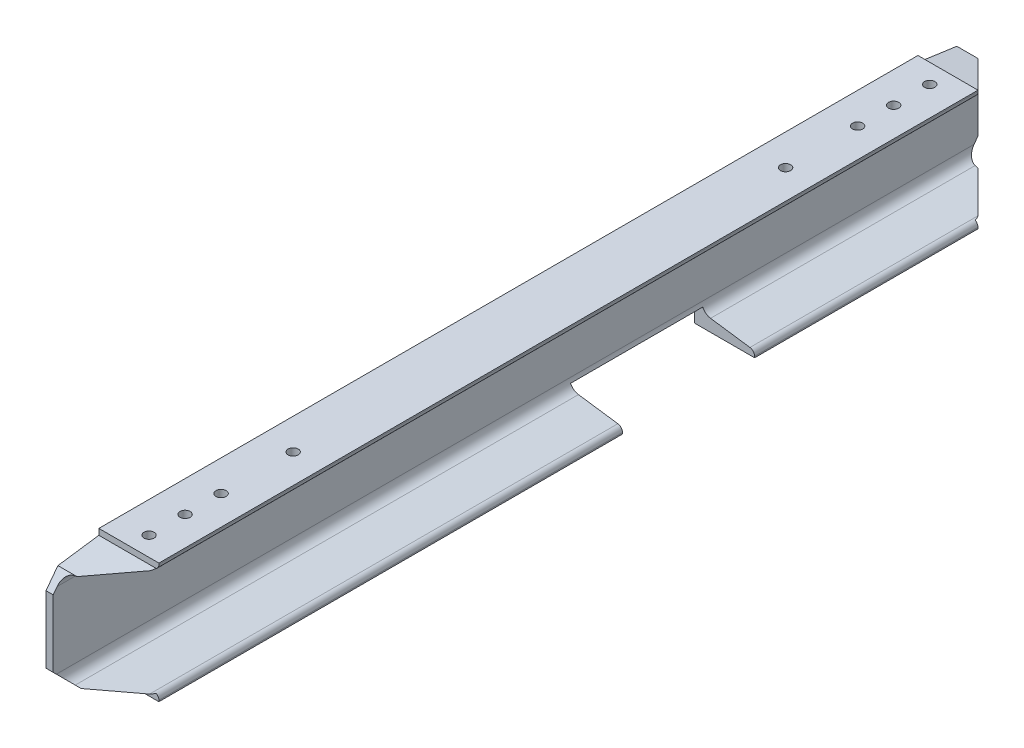
from build123d import *
from OCP.BRepFilletAPI import BRepFilletAPI_MakeChamfer

# Parameters (mm, degrees)
BOSS_EXTRUDE1_DEPTH    = 694
SKETCH3_W              = 110
SKETCH3_H              = 70.171613021
CUT_EXTRUDE1_DEPTH     = 145
M10_TAPPED_HOLE2_D     = 8.5
M10_TAPPED_HOLE2_DEPTH = 24.5
M10_TAPPED_HOLE2_TIP   = 2.553657631
BOSS_EXTRUDE2_START    = 44
BOSS_EXTRUDE2_DEPTH    = 44
BOSS_EXTRUDE3_DEPTH    = 44
CUT_EXTRUDE3_DEPTH     = 100
CHAMFER1_SIZE          = 10
CHAMFER1_SIZE2         = 11.749570117
M6_TAPPED_HOLE1_D      = 5
M6_TAPPED_HOLE1_DEPTH  = 15
M6_TAPPED_HOLE1_TIP    = 1.502151548


with BuildPart() as part:
    # Sketch1 → Boss-Extrude1 (new body)
    with BuildSketch(Plane.XY):
        with BuildLine():
            Line((0, 0), (0, -100))
            Line((0, -100), (50, -100))
            Line((50, -100), (50, -98.925311188))
            ThreePointArc((50, -98.925311188), (48.896193111, -95.973045557), (46.126278954, -94.469104878))
            Line((46.126278954, -94.469104878), (13.317028642, -89.858065454))
            ThreePointArc((13.317028642, -89.858065454), (8.084968568, -87.017288616), (6, -81.440786869))
            Line((6, -81.440786869), (6, -18.559213131))
            ThreePointArc((6, -18.559213131), (8.084968568, -12.982711384), (13.317028642, -10.141934546))
            Line((13.317028642, -10.141934546), (46.126278954, -5.530895122))
            ThreePointArc((46.126278954, -5.530895122), (48.896193111, -4.026954443), (50, -1.074688812))
            Line((50, -1.074688812), (50, 0))
            Line((50, 0), (0, 0))
        make_face()
    extrude(amount=BOSS_EXTRUDE1_DEPTH)

    # Sketch3 → Cut-Extrude1 (cut)
    with BuildSketch(Plane.ZY):
        with Locations((247, -120.085806511)):
            Rectangle(SKETCH3_W, SKETCH3_H)
    extrude(amount=-CUT_EXTRUDE1_DEPTH, mode=Mode.SUBTRACT)

    # M10 Tapped Hole2
    with Locations(Plane(origin=(0, 0, 0), x_dir=(1, 0, 0), z_dir=(0, 1, 0))):
        with Locations((25.782416052, -142), (25.782416052, -82), (25.782416052, -22), (25.782416052, -52), (25.782416052, -552), (25.782416052, -612), (25.782416052, -642), (25.782416052, -672)):
            Hole(M10_TAPPED_HOLE2_D / 2, depth=M10_TAPPED_HOLE2_DEPTH)
            with Locations((0, 0, -(M10_TAPPED_HOLE2_DEPTH + M10_TAPPED_HOLE2_TIP / 2))):  # 118° drill point
                Cone(0, M10_TAPPED_HOLE2_D / 2, M10_TAPPED_HOLE2_TIP, mode=Mode.SUBTRACT)

    # Sketch15 → Boss-Extrude2 (add)
    with BuildSketch(Plane(origin=(0, 0, 0), x_dir=(-1, 0, 0), z_dir=(0, 0, -1)).offset(BOSS_EXTRUDE2_START)):
        with BuildLine():
            Line((0, 0), (-50, 0))
            Line((-50, 0), (-50, -1.074688812))
            ThreePointArc((-50, -1.074688812), (-48.896193111, -4.026954443), (-46.126278954, -5.530895122))
            Line((-46.126278954, -5.530895122), (-13.317028642, -10.141934546))
            ThreePointArc((-13.317028642, -10.141934546), (-8.084968568, -12.982711384), (-6, -18.559213131))
            Line((-6, -18.559213131), (-6, -81.440786869))
            ThreePointArc((-6, -81.440786869), (-8.084968568, -87.017288616), (-13.317028642, -89.858065454))
            Line((-13.317028642, -89.858065454), (-46.126278954, -94.469104878))
            ThreePointArc((-46.126278954, -94.469104878), (-48.896193111, -95.973045557), (-50, -98.925311188))
            Line((-50, -98.925311188), (-50, -100))
            Line((-50, -100), (0, -100))
            Line((0, -100), (0, 0))
        make_face()
    extrude(amount=-BOSS_EXTRUDE2_DEPTH)

    # Sketch17 → Boss-Extrude3 (add)
    with BuildSketch(Plane.XY.offset(694)):
        with BuildLine():
            Line((50, 0), (0, 0))
            Line((0, 0), (0, -100))
            Line((0, -100), (50, -100))
            Line((50, -100), (50, -98.925311188))
            ThreePointArc((50, -98.925311188), (48.896193111, -95.973045557), (46.126278954, -94.469104878))
            Line((46.126278954, -94.469104878), (13.317028642, -89.858065454))
            ThreePointArc((13.317028642, -89.858065454), (8.084968568, -87.017288616), (6, -81.440786869))
            Line((6, -81.440786869), (6, -18.559213131))
            ThreePointArc((6, -18.559213131), (8.084968568, -12.982711384), (13.317028642, -10.141934546))
            Line((13.317028642, -10.141934546), (46.126278954, -5.530895122))
            ThreePointArc((46.126278954, -5.530895122), (48.896193111, -4.026954443), (50, -1.074688812))
            Line((50, -1.074688812), (50, 0))
        make_face()
    extrude(amount=BOSS_EXTRUDE3_DEPTH)

    # Sketch16 → Cut-Extrude3 (cut)
    with BuildSketch(Plane.ZY):
        Polygon((6, -100), (-44, -100), (-44, 0), (6, 0), (6, -4.986479132), (-38, -11.170275859), (-38, -88.829724141), (6, -95.013520868), align=None)
        Polygon((688, -95.013520868), (688, -100), (738, -100), (738, 0), (688, 0), (688, -4.986479132), (732, -11.170275859), (732, -88.829724141), align=None)
    extrude(amount=-CUT_EXTRUDE3_DEPTH, mode=Mode.SUBTRACT)

    # Chamfer1: one chamfer whose edges measure the first distance from different faces: ONE call of the kernel's chamfer builder (chamfer() names one face for all edges)
    chamfer1_edges_1 = [part.edges().sort_by_distance(p)[0] for p in [
        (5.149190275, -11.170275859, 732),
    ]]
    chamfer1_side_1 = [part.faces().sort_by_distance(p)[0] for p in [
        (16.706788041, -7.313969364, 704.560953522),
    ]]
    chamfer1_edges_2 = [part.edges().sort_by_distance(p)[0] for p in [
        (5.149190275, -88.829724141, 732),
    ]]
    chamfer1_side_2 = [part.faces().sort_by_distance(p)[0] for p in [
        (3.160002327, -50, 732),
    ]]
    chamfer1_edges_3 = [part.edges().sort_by_distance(p)[0] for p in [
        (5.149190275, -11.170275859, -38),
    ]]
    chamfer1_side_3 = [part.faces().sort_by_distance(p)[0] for p in [
        (3.160002327, -50, -38),
    ]]
    chamfer1_edges_4 = [part.edges().sort_by_distance(p)[0] for p in [
        (5.149190275, -88.829724141, -38),
    ]]
    chamfer1_side_4 = [part.faces().sort_by_distance(p)[0] for p in [
        (16.706788041, -92.686030636, -10.560953522),
    ]]
    chamfer1 = BRepFilletAPI_MakeChamfer(part.part.solid().wrapped)
    for e in chamfer1_edges_1:
        chamfer1.Add(CHAMFER1_SIZE, CHAMFER1_SIZE2, e.wrapped, chamfer1_side_1[0].wrapped)  # the first distance lies on this face
    for e in chamfer1_edges_2:
        chamfer1.Add(CHAMFER1_SIZE, CHAMFER1_SIZE2, e.wrapped, chamfer1_side_2[0].wrapped)  # the first distance lies on this face
    for e in chamfer1_edges_3:
        chamfer1.Add(CHAMFER1_SIZE, CHAMFER1_SIZE2, e.wrapped, chamfer1_side_3[0].wrapped)  # the first distance lies on this face
    for e in chamfer1_edges_4:
        chamfer1.Add(CHAMFER1_SIZE, CHAMFER1_SIZE2, e.wrapped, chamfer1_side_4[0].wrapped)  # the first distance lies on this face
    add(Compound.cast(chamfer1.Shape()), mode=Mode.REPLACE)

    # M6 Tapped Hole1
    with Locations(Plane.ZY):
        with Locations((334.5, -20), (359.5, -20)):
            Hole(M6_TAPPED_HOLE1_D / 2, depth=M6_TAPPED_HOLE1_DEPTH)
            with Locations((0, 0, -(M6_TAPPED_HOLE1_DEPTH + M6_TAPPED_HOLE1_TIP / 2))):  # 118° drill point
                Cone(0, M6_TAPPED_HOLE1_D / 2, M6_TAPPED_HOLE1_TIP, mode=Mode.SUBTRACT)


solid = part.part
